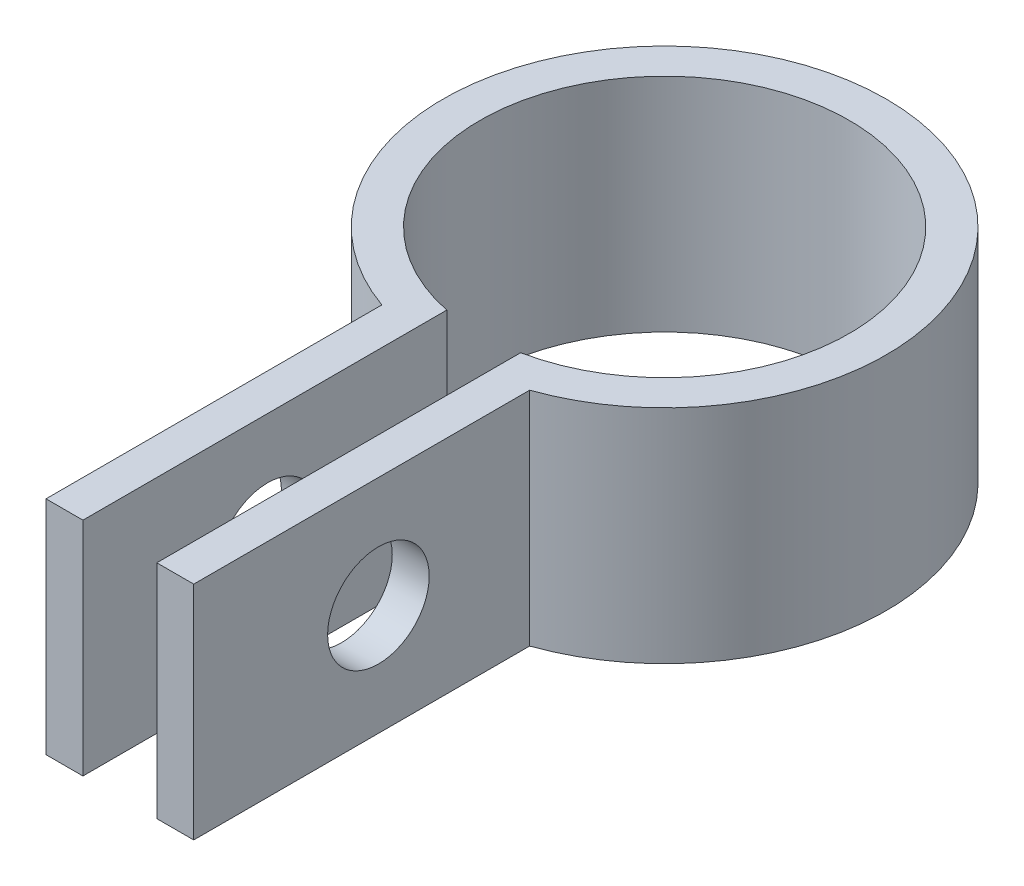
SolidWorks part; units mm, degrees
material "普通碳钢"
ref_plane "前视基准面" through (0, 0, 0) normal (0, 0, 1) x (1, 0, 0)
ref_plane "上视基准面" through (0, 0, 0) normal (0, 1, 0) x (1, 0, 0)
ref_plane "右视基准面" through (0, 0, 0) normal (1, 0, 0) x (0, 0, -1)
sketch "草图1" plane through (0, 0, 0) normal (0, 1, 0) x (1, 0, 0)
  line L0 (-19.4252, 0) -> (19.303, 0) construction
  line L1 (0, 30.6039) -> (0, -22.4184) construction
  line L2 (8, -59) -> (4, -59)
  line L3 (8, -22.6274) -> (8, -59)
  line L4 (-8, -22.6274) -> (-8, -59)
  line L5 (-8, -59) -> (-4, -59)
  line L6 (-4, -19.5959) -> (-4, -59)
  line L7 (4, -19.5959) -> (4, -59)
  arc A0 (4, -19.5959) -> (-4, -19.5959) centre (0, 0) ccw
  arc A2 (8, -22.6274) -> (-8, -22.6274) centre (0, 0) ccw
  dimension "D1" = 40
  dimension "D2" = 24
  dimension "D3" = 59
  dimension "D4" = 8
  dimension "D5" = 16
extrude "凸台-拉伸1" add sketch "草图1" along normal mid plane 24
sketch "草图2" plane through (0, 0, 0) normal (1, 0, 0) x (0, 0, -1)
  line L0 (-73.8393, 0) -> (35.7564, 0) construction
  line L1 (0, 55.6064) -> (0, -32.709) construction
  circle A0 centre (-39, 0) radius 5.5
  dimension "D2" = 11
  dimension "D1" = 39
extrude "切除-拉伸1" cut sketch "草图2" against normal through all both and the other way through all
